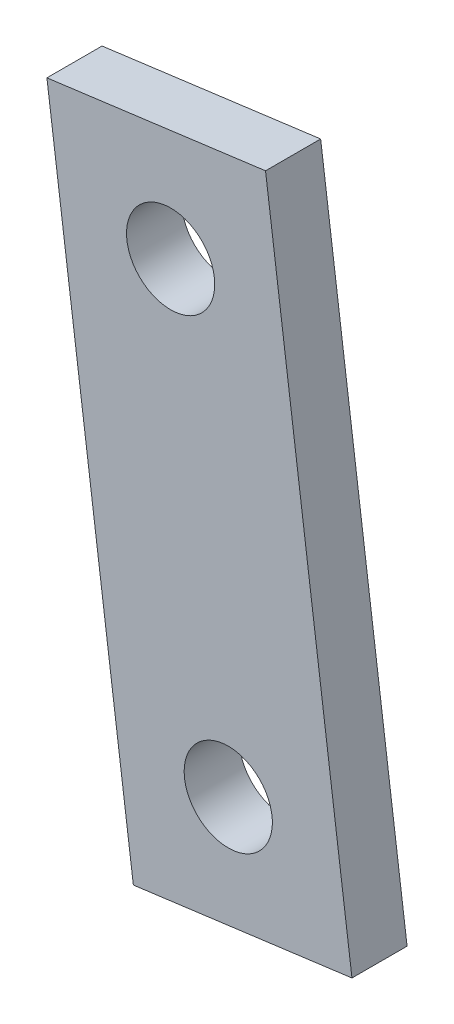
from build123d import *

# Parameters (mm, degrees)
SKETCH1_R           = 8
BOSS_EXTRUDE1_DEPTH = 10


with BuildPart() as part:
    # Sketch1 → Boss-Extrude1 (new body)
    with BuildSketch(Plane.XY):
        Polygon((5137.305231976, 2244.717137192), (5129.46700669, 2304.202952513), (5169.124216904, 2309.428436037), (5184.800667476, 2190.456805396), (5145.143457262, 2185.231321872), align=None)
        with Locations((5151.908353559, 2286.987089168)):
            Circle(SKETCH1_R, mode=Mode.SUBTRACT)
        with Locations(Location((5162.359320607, 2207.67266874, 0), (0, 0, 180))):
            Circle(SKETCH1_R, mode=Mode.SUBTRACT)
    extrude(amount=BOSS_EXTRUDE1_DEPTH)


solid = part.part
